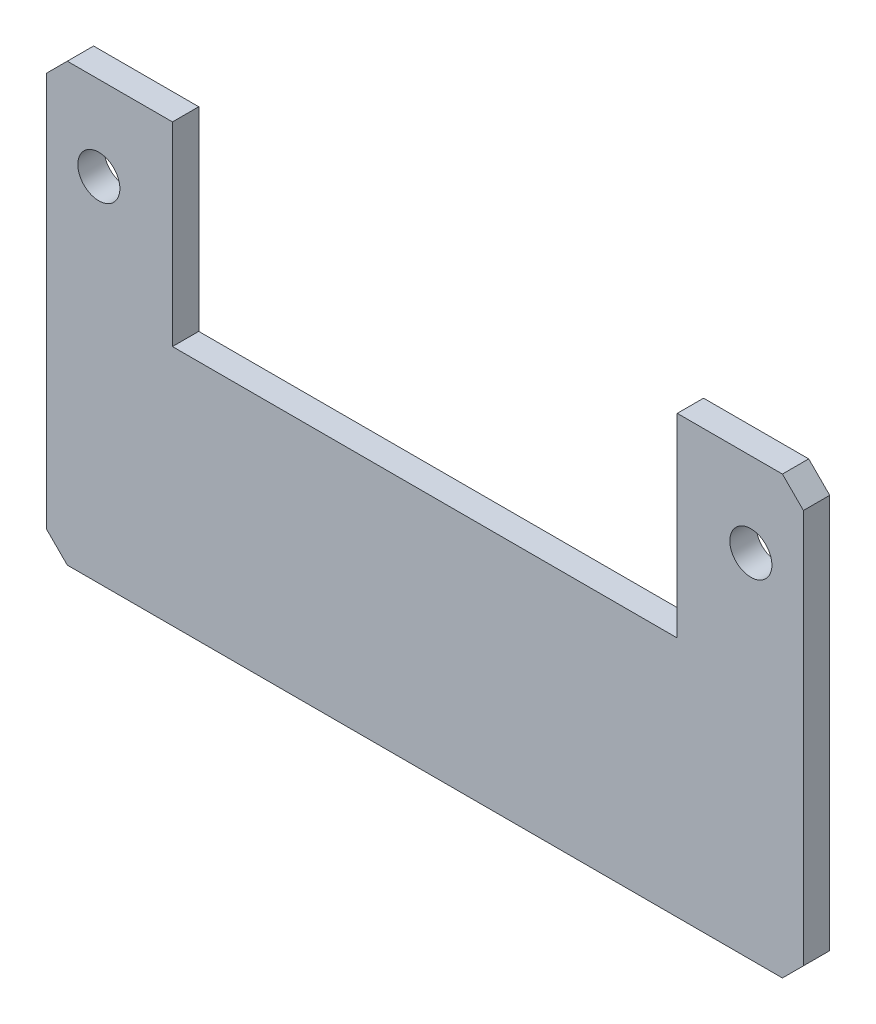
from build123d import *

# Parameters (mm, degrees)
SKETCH1_R           = 20
BOSS_EXTRUDE1_DEPTH = 25
CHAMFER1_SIZE       = 20


with BuildPart() as part:
    # Sketch1 → Boss-Extrude1 (new body)
    with BuildSketch(Plane.XY):
        Polygon((120, 0), (0, 0), (0, -415), (720, -415), (720, 0), (600, 0), (600, -185), (120, -185), align=None)
        with Locations((50, -80)):
            Circle(SKETCH1_R, mode=Mode.SUBTRACT)
        with Locations((670, -80)):
            Circle(SKETCH1_R, mode=Mode.SUBTRACT)
    extrude(amount=BOSS_EXTRUDE1_DEPTH)

    # Chamfer1
    chamfer1_edges = [part.edges().sort_by_distance(p)[0] for p in [
        (720, 0, 12.5),
        (720, -415, 12.5),
        (0, -415, 12.5),
        (0, 0, 12.5),
    ]]
    chamfer(chamfer1_edges, length=CHAMFER1_SIZE)


solid = part.part
